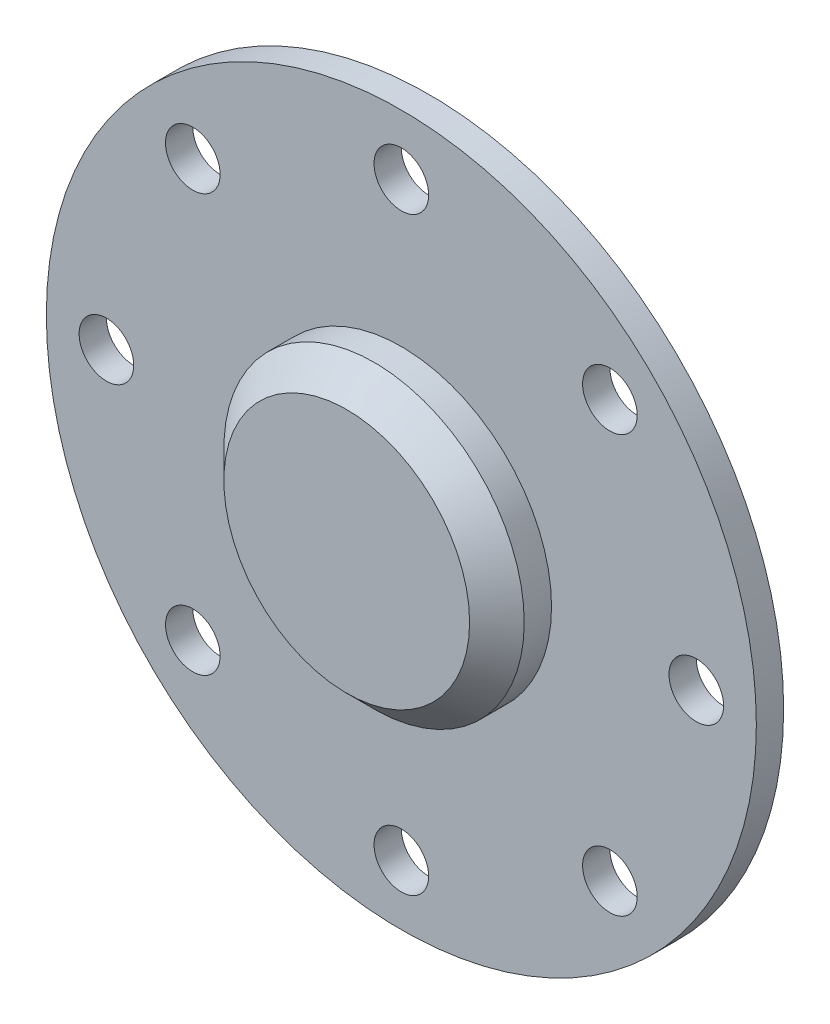
SolidWorks part; units mm, degrees
material "灰铸铁"
ref_plane "前视基准面" through (0, 0, 0) normal (0, 0, 1) x (1, 0, 0)
ref_plane "上视基准面" through (0, 0, 0) normal (0, 1, 0) x (1, 0, 0)
ref_plane "右视基准面" through (0, 0, 0) normal (1, 0, 0) x (0, 0, -1)
sketch "草图1" plane through (0, 0, 0) normal (0, 0, 1) x (1, 0, 0)
  circle A0 centre (0, 0) radius 130
  circle A1 centre (0, 0) radius 108 construction
  circle A2 centre (0, 108) radius 10
  circle A3 centre (76.3675, 76.3675) radius 10
  circle A4 centre (108, 0) radius 10
  circle A5 centre (76.3675, -76.3675) radius 10
  circle A6 centre (0, -108) radius 10
  circle A7 centre (-76.3675, -76.3675) radius 10
  circle A8 centre (-108, 0) radius 10
  circle A9 centre (-76.3675, 76.3675) radius 10
  point P22 (0, 0)
  dimension "D1" = 8
extrude "凸台-拉伸1" add sketch "草图1" along normal blind 10
sketch "草图2" plane through (0, 0, 10) normal (0, 0, 1) x (1, 0, 0)
  circle A0 centre (0, 0) radius 55
extrude "凸台-拉伸2" add sketch "草图2" along normal blind 20
sketch "草图3" plane through (0, 0, 0) normal (0, 0, -1) x (-1, 0, 0)
  circle A0 centre (0, 0) radius 45
extrude "切除-拉伸1" cut sketch "草图3" against normal blind 20
chamfer "倒角1" distance 10 angle 45 1 edges at (55, 0, 30)
